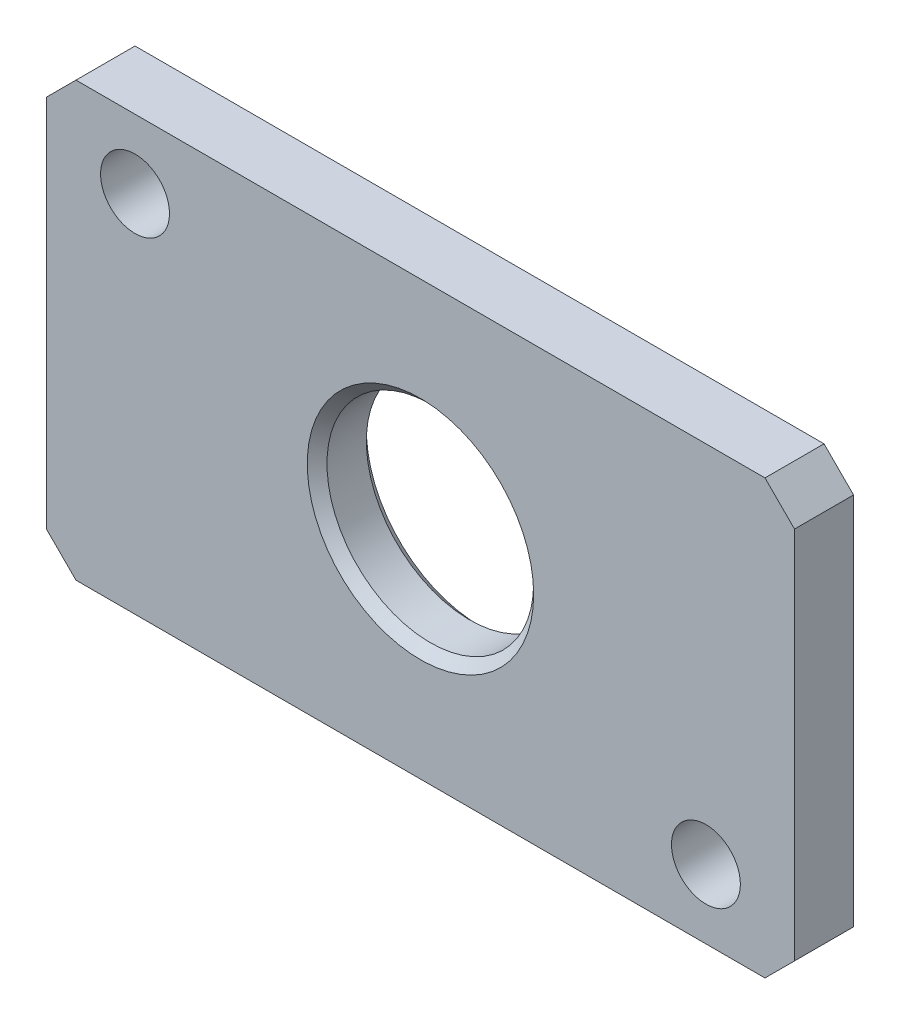
SolidWorks part; units mm, degrees
material "SUS304"
ref_plane "Front Plane" through (0, 0, 0) normal (0, 0, 1) x (1, 0, 0)
ref_plane "Top Plane" through (0, 0, 0) normal (0, 1, 0) x (1, 0, 0)
ref_plane "Right Plane" through (0, 0, 0) normal (1, 0, 0) x (0, 0, -1)
sketch "Sketch1" plane through (0, 0, 0) normal (0, 0, 1) x (1, 0, 0)
  line L1 (-19, 11) -> (19, 11)
  line L2 (-19, 11) -> (-19, -11)
  line L3 (-19, -11) -> (19, -11)
  line L4 (19, 11) -> (19, -11)
  line L5 (-19, 11) -> (19, -11) construction
  line L6 (-19, -11) -> (19, 11) construction
  circle A0 centre (0, 0) radius 5.25
  circle A1 centre (-14.5, 7.5) radius 1.75
  circle A2 centre (14.5, -7.5) radius 1.75
  point P0 (0, 0)
  dimension "D3" = 10.5
  dimension "D4" = 15
  dimension "D6" = 29
  dimension "D8" = 3.5
  dimension "D1" = 38
  dimension "D2" = 22
  dimension "D5" = 7.5
  dimension "D7" = 14.5
extrude "Boss-Extrude1" add sketch "Sketch1" along normal blind 3
chamfer "Chamfer1" distance 1.5 angle 45 4 edges at (19, 11, 1.5) (19, -11, 1.5) (-19, -11, 1.5) (-19, 11, 1.5)
chamfer "Chamfer2" distance 0.5 angle 45 2 edges at (5.25, 0, 0) (5.25, 0, 3)
